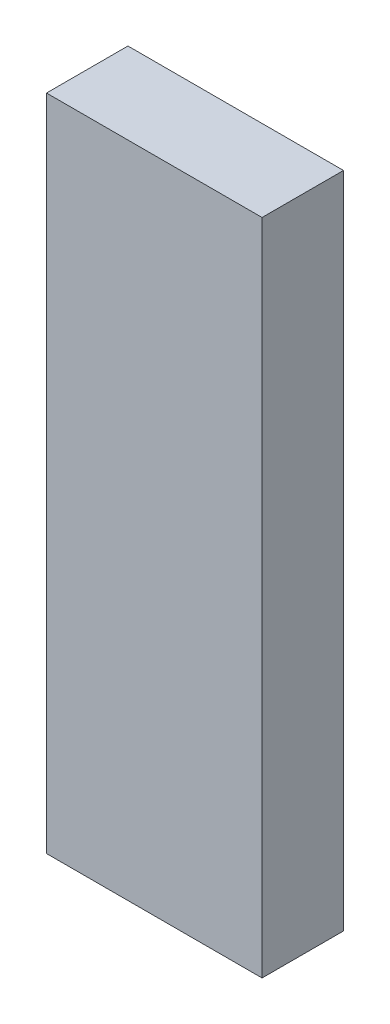
SolidWorks part; units mm, degrees
ref_plane "前视基准面" through (0, 0, 0) normal (0, 0, 1) x (1, 0, 0)
ref_plane "上视基准面" through (0, 0, 0) normal (0, 1, 0) x (1, 0, 0)
ref_plane "右视基准面" through (0, 0, 0) normal (1, 0, 0) x (0, 0, -1)
sketch "草图1" plane through (0, 0, 0) normal (0, 0, 1) x (1, 0, 0)
  line L1 (-45, -137.5) -> (45, -137.5)
  line L2 (-45, -137.5) -> (-45, 137.5)
  line L3 (-45, 137.5) -> (45, 137.5)
  line L4 (45, -137.5) -> (45, 137.5)
  line L5 (-45, -137.5) -> (45, 137.5) construction
  line L6 (-45, 137.5) -> (45, -137.5) construction
  point P0 (0, 0)
  dimension "D1" = 275
  dimension "D2" = 90
extrude "凸台-拉伸1" add sketch "草图1" along normal blind 34
